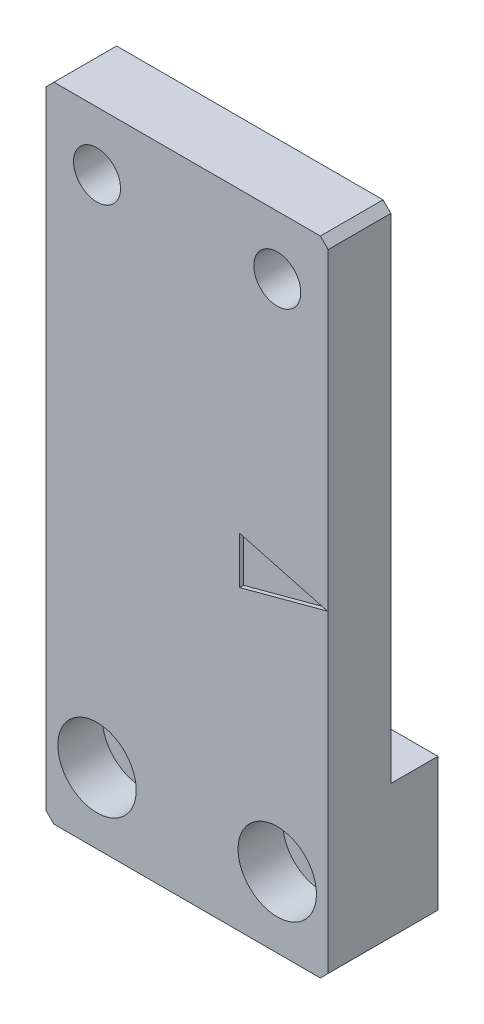
SolidWorks part; units mm, degrees
material "A5052"
ref_plane "Front Plane" through (0, 0, 0) normal (0, 0, 1) x (1, 0, 0)
ref_plane "Top Plane" through (0, 0, 0) normal (0, 1, 0) x (1, 0, 0)
ref_plane "Right Plane" through (0, 0, 0) normal (1, 0, 0) x (0, 0, -1)
sketch "Sketch1" plane through (0, 0, 0) normal (1, 0, 0) x (0, 0, -1)
  line L0 (14, 0) -> (0, 0)
  line L1 (0, 0) -> (0, 82)
  line L2 (0, 82) -> (8, 82)
  line L3 (8, 82) -> (8, 18)
  line L4 (8, 18) -> (14, 18)
  line L5 (14, 18) -> (14, 0)
  dimension "D1" = 82
  dimension "D2" = 18
  dimension "D3" = 14
  dimension "D4" = 8
extrude "Boss-Extrude1" add sketch "Sketch1" along normal mid plane 36
hole_wizard "Hole size per socket head cap screw type1" positions "Sketch4" profile "Sketch3" counterbore size "M5" standard "GB" end condition through all
sketch "Sketch4" plane through (0, 0, 0) normal (0, 0, 1) x (1, 0, 0)
  line L0 (0, 0) -> (0, 5.1243) construction
  line L2 (18, 0) -> (-18, 0) construction
  point P0 (11.5, 9)
  point P1 (-11.5, 9)
  dimension "D1" = 23
  dimension "D2" = 9
sketch "Sketch3" plane through (11.5, 9, 0) normal (1, 0, 0) x (0, -1, 0)
  line L0 (0, 0) -> (0, 14)
  line L1 (0, 14) -> (2.75, 14)
  line L3 (2.75, 14) -> (2.75, 5.7)
  line L4 (2.75, 5.7) -> (5, 5.7)
  line L5 (5, 5.7) -> (5, 0)
  line L7 (5, 0) -> (0, 0)
  line L11 (0, -6.35) -> (0, 107.95) construction
  dimension "通孔孔直径" = 5.5
  dimension "通孔孔深度" = 14
  dimension "柱形沉头孔直径" = 10
  dimension "柱形沉头孔深度" = 5.7
sketch "Sketch5" plane through (0, 0, 0) normal (0, 0, 1) x (1, 0, 0)
  line L0 (0, 0) -> (0, 11.4795) construction
  line L1 (18, 82) -> (-18, 82) construction
  circle A0 centre (-11.5, 74.5) radius 3
  circle A1 centre (11.5, 74.5) radius 3
  dimension "D1" = 6
  dimension "D2" = 23
  dimension "D3" = 7.5
extrude "Cut-Extrude1" cut sketch "Sketch5" against normal through all
chamfer "Chamfer1" distance 1 angle 45 4 edges at (-18, 0, -7) (18, 0, -7) (18, 82, -4) (-18, 82, -4)
sketch "Sketch6" plane through (0, 0, 0) normal (0, 0, 1) x (1, 0, 0)
  line L0 (6.7, 44) -> (17.8962, 41)
  line L1 (18, 81) -> (18, 1) construction
  line L2 (17.8962, 41) -> (6.7, 38)
  line L3 (6.7, 38) -> (6.7, 44)
  line L4 (17.8962, 41) -> (11.5816, 41) construction
  point P9 (18, 41)
  dimension "D1" = 15
  dimension "D2" = 11.3
  dimension "D3" = 6
extrude "Cut-Extrude3" cut sketch "Sketch6" against normal blind 0.5
